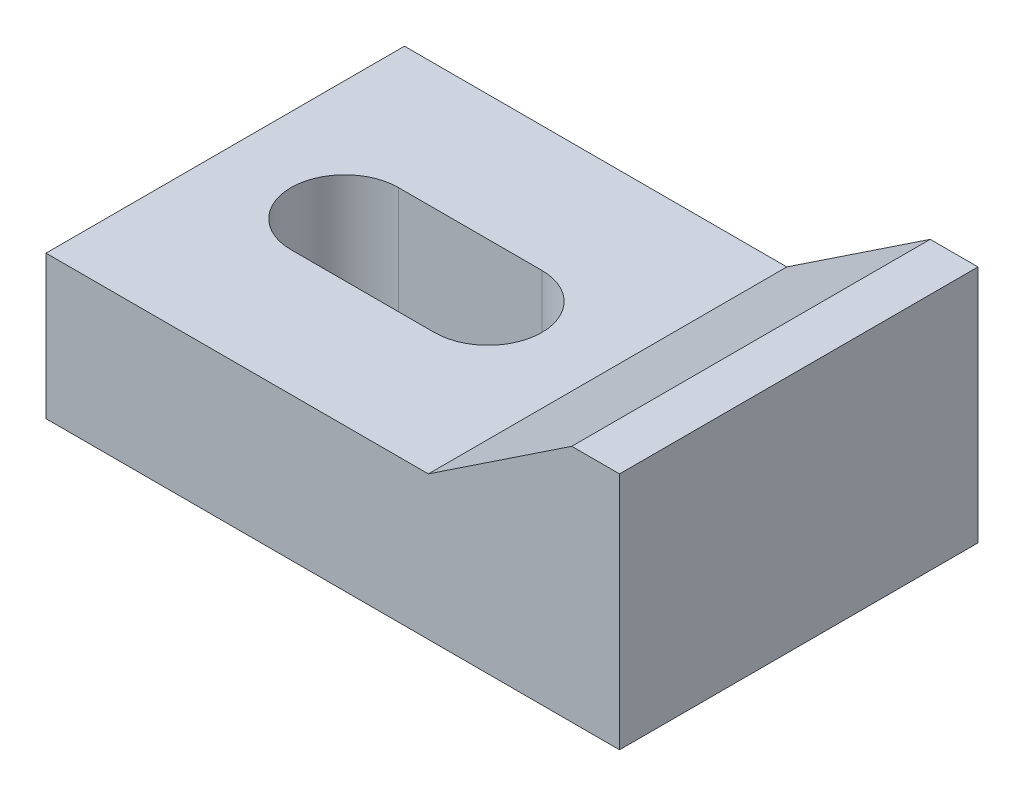
SolidWorks part; units mm, degrees
material "锡轴承青铜"
ref_plane "Front Plane" through (0, 0, 0) normal (0, 0, 1) x (1, 0, 0)
ref_plane "Top Plane" through (0, 0, 0) normal (0, 1, 0) x (1, 0, 0)
ref_plane "Right Plane" through (0, 0, 0) normal (1, 0, 0) x (0, 0, -1)
sketch "Sketch1" plane through (0, 0, 0) normal (0, 0, 1) x (1, 0, 0)
  line L0 (-12, 1) -> (4, 1)
  line L1 (-12, -5) -> (12, -5)
  line L2 (-12, -5) -> (-12, 5)
  line L3 (-12, 5) -> (12, 5)
  line L4 (12, -5) -> (12, 5)
  line L5 (-12, -5) -> (12, 5) construction
  line L6 (-12, 5) -> (12, -5) construction
  line L7 (4, 1) -> (10, 5)
  point P0 (0, 0)
  dimension "D1" = 24
  dimension "D2" = 10
  dimension "D3" = 2
  dimension "D4" = 6
  dimension "D5" = 16
extrude "Boss-Extrude1" add sketch "Sketch1" along normal mid plane 15 contours L7 L0 L2 L1 L4 L3
sketch "Sketch2" plane through (0, 1, 0) normal (0, 1, 0) x (1, 0, 0)
  line L0 (4, 0) -> (-12, 0) construction
  line L1 (4, -7.5) -> (4, 7.5) construction
  line L2 (-12, -7.5) -> (-12, 7.5) construction
  line L3 (-7, 0) -> (-1, 0) construction
  line L4 (-7, 2.25) -> (-1, 2.25)
  line L5 (-7, -2.25) -> (-1, -2.25)
  arc A0 (-7, 2.25) -> (-7, -2.25) centre (-7, 0) ccw
  arc A1 (-1, -2.25) -> (-1, 2.25) centre (-1, 0) ccw
  point P8 (-4, 0)
  dimension "D1" = 4.5
  dimension "D2" = 6
extrude "Cut-Extrude1" cut sketch "Sketch2" against normal up to next
